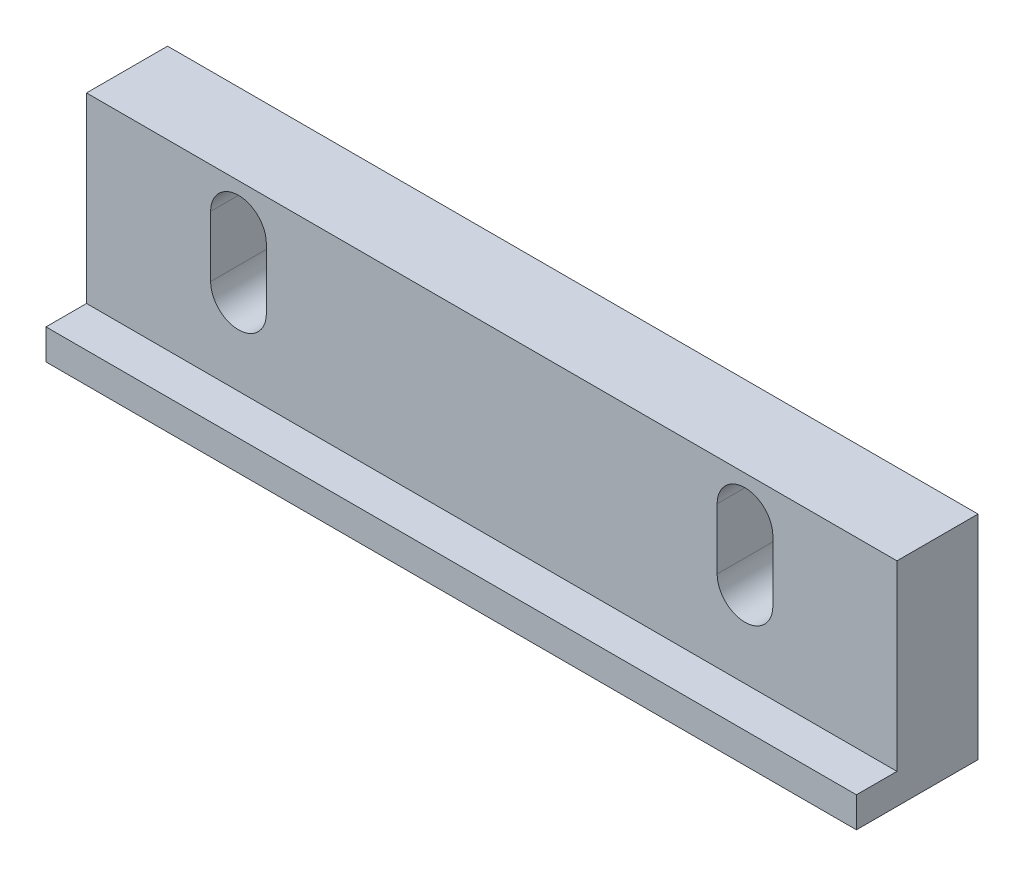
SolidWorks part; units mm, degrees
ref_plane "前视基准面" through (0, 0, 0) normal (0, 0, 1) x (1, 0, 0)
ref_plane "上视基准面" through (0, 0, 0) normal (0, 1, 0) x (1, 0, 0)
ref_plane "右视基准面" through (0, 0, 0) normal (1, 0, 0) x (0, 0, -1)
sketch "草图1" plane through (0, 0, 0) normal (0, 0, 1) x (1, 0, 0)
  line L1 (-40, 21) -> (40, 21)
  line L2 (-40, 21) -> (-40, 0)
  line L3 (-40, 0) -> (40, 0)
  line L4 (40, 21) -> (40, 0)
  dimension "D1" = 80
  dimension "D2" = 21
extrude "凸台-拉伸1" add sketch "草图1" along normal blind 8
sketch "草图2" plane through (0, 0, 8) normal (0, 0, 1) x (1, 0, 0)
  line L0 (40, 0) -> (40, 21) construction
  line L1 (-40, 0) -> (40, 0)
  line L2 (-40, 0) -> (-40, 3)
  line L3 (-40, 3) -> (40, 3)
  line L4 (40, 0) -> (40, 3)
  dimension "D1" = 3
extrude "凸台-拉伸2" add sketch "草图2" along normal blind 4
sketch "草图3" plane through (0, 0, 8) normal (0, 0, 1) x (1, 0, 0)
  line L0 (-25, 17) -> (-25, 11) construction
  line L1 (-22.25, 17) -> (-22.25, 11)
  line L2 (-27.75, 17) -> (-27.75, 11)
  line L3 (40, 21) -> (-40, 21) construction
  line L4 (-40, 21) -> (-40, 3) construction
  arc A0 (-22.25, 17) -> (-27.75, 17) centre (-25, 17) ccw
  arc A1 (-27.75, 11) -> (-22.25, 11) centre (-25, 11) ccw
  point P2 (-25, 14)
  dimension "D1" = 2.75
  dimension "D3" = 4
  dimension "D4" = 15
  dimension "D2" = 6
extrude "切除-拉伸1" cut sketch "草图3" against normal blind 8
ref_plane "基准面1" through (0, 0, 0) normal (-1, 0, 0) x (0, 0, 1)
mirror "镜向1" about plane through (0, 0, 0) normal (-1, 0, 0) of "切除-拉伸1"
